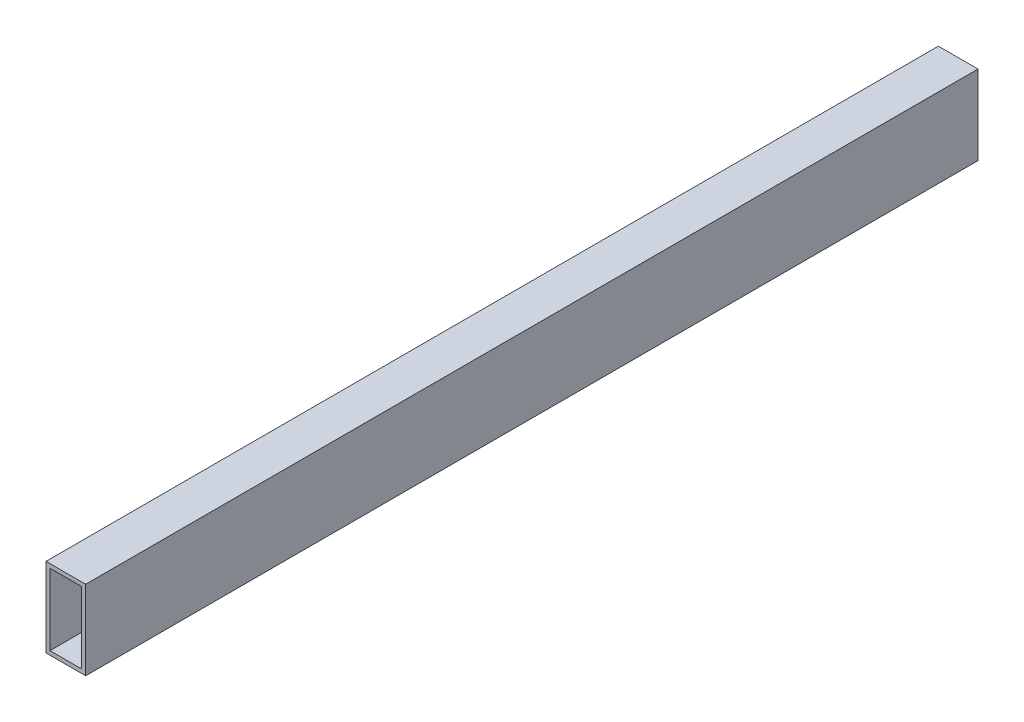
SolidWorks part; units mm, degrees
ref_plane "前视基准面" through (0, 0, 0) normal (0, 0, 1) x (1, 0, 0)
ref_plane "上视基准面" through (0, 0, 0) normal (0, 1, 0) x (1, 0, 0)
ref_plane "右视基准面" through (0, 0, 0) normal (1, 0, 0) x (0, 0, -1)
other "Configuration Table"
sketch "草图1" plane through (0, 0, 0) normal (0, 0, 1) x (1, 0, 0)
  line L0 (-20, -40) -> (20, -40)
  line L1 (20, -40) -> (20, 40)
  line L2 (20, 40) -> (-20, 40)
  line L3 (-20, 40) -> (-20, -40)
  line L4 (-16, -36) -> (16, -36)
  line L5 (16, -36) -> (16, 36)
  line L6 (16, 36) -> (-16, 36)
  line L7 (-16, 36) -> (-16, -36)
  point P0 (0, 0)
  dimension "D1" = 4
  dimension "D2" = 20
  dimension "D3" = 36
  dimension "D4" = 40
  dimension "D5" = 4
  dimension "D6" = 40
  dimension "D7" = 76
  dimension "D8" = 80
extrude "凸台-拉伸1" add sketch "草图1" against normal mid plane 900
